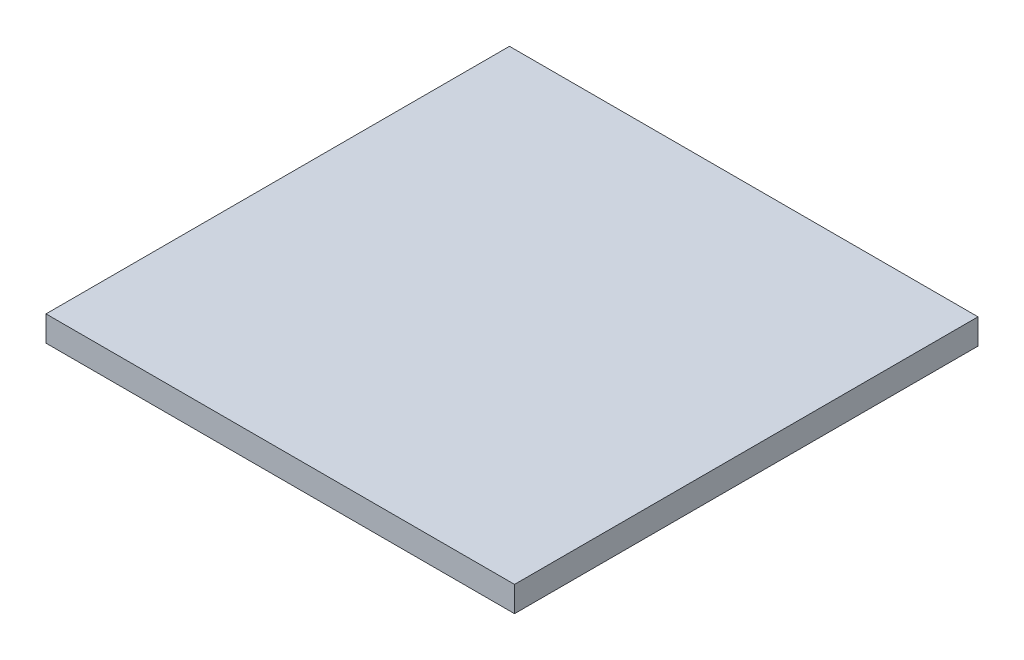
SolidWorks part; units mm, degrees
ref_plane "Front Plane" through (0, 0, 0) normal (0, 0, 1) x (1, 0, 0)
ref_plane "Top Plane" through (0, 0, 0) normal (0, 1, 0) x (1, 0, 0)
ref_plane "Right Plane" through (0, 0, 0) normal (1, 0, 0) x (0, 0, -1)
sketch "Sketch1" plane through (0, 0, 0) normal (0, 1, 0) x (1, 0, 0)
  line L1 (0, 0) -> (-369, 0)
  line L2 (0, 0) -> (0, 365)
  line L3 (0, 365) -> (-369, 365)
  line L4 (-369, 0) -> (-369, 365)
  dimension "D1" = 369
  dimension "D2" = 365
extrude "Boss-Extrude1" add sketch "Sketch1" along normal blind 20
